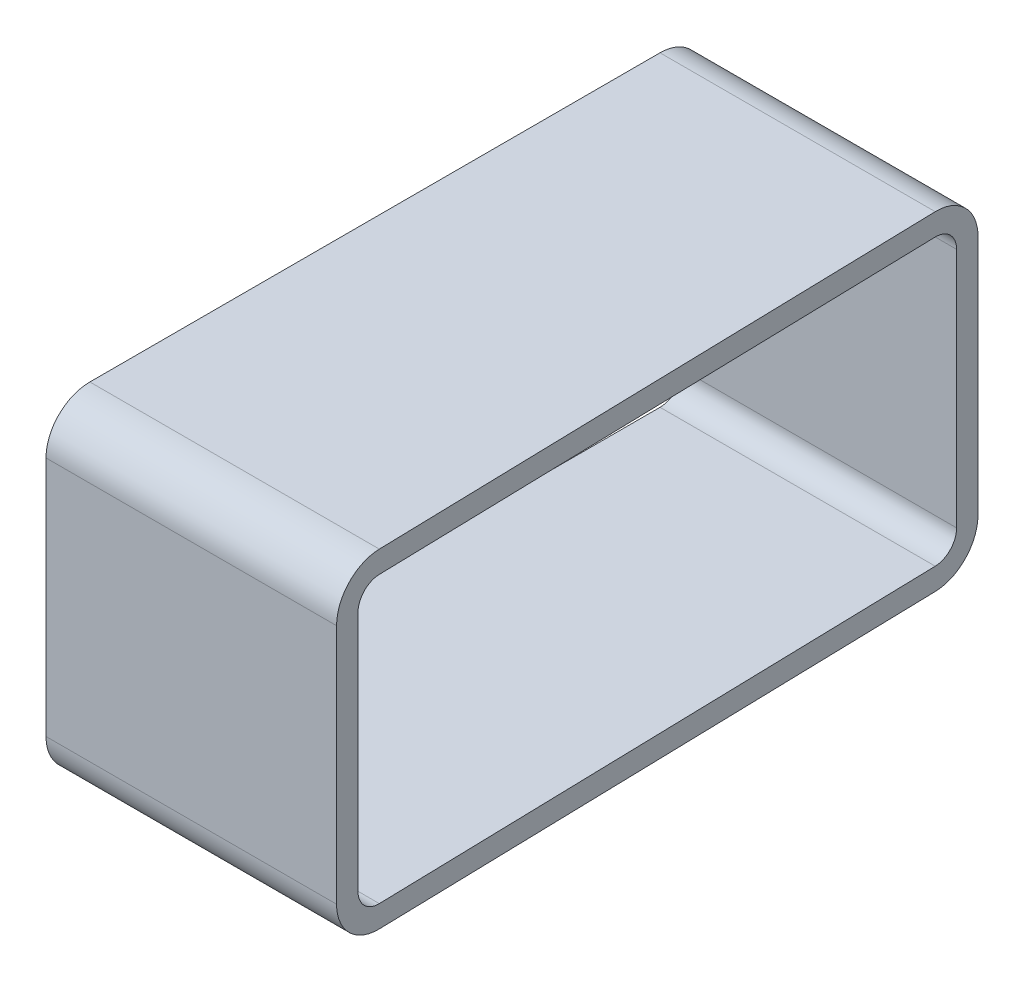
SolidWorks part; units mm, degrees
material "普通碳钢"
ref_plane "Front Plane" through (0, 0, 0) normal (0, 0, 1) x (1, 0, 0)
ref_plane "Top Plane" through (0, 0, 0) normal (0, 1, 0) x (1, 0, 0)
ref_plane "Right Plane" through (0, 0, 0) normal (1, 0, 0) x (0, 0, -1)
other "Configuration Table"
sketch "草图1" plane through (0, 0, 0) normal (0, 0, 1) x (1, 0, 0)
  line L0 (0, 0) -> (53, 0)
  dimension "D1" = 53
other "GB/6728-1986 rectangular hollow section 120 X 60 X 4(1)"
ref_plane "Plane1" through (0, 0, 0) normal (1, 0, 0) x (0, 1, 0)
sketch "Sketch1" plane through (0, 0, 0) normal (1, 0, 0) x (0, 1, 0)
  line L0 (-22, -56) -> (22, -56)
  line L1 (-26, -52) -> (-26, 52)
  line L2 (22, 56) -> (-22, 56)
  line L3 (26, 52) -> (26, -52)
  line L4 (-22, -60) -> (22, -60)
  line L5 (-30, -52) -> (-30, 52)
  line L6 (22, 60) -> (-22, 60)
  line L7 (30, 52) -> (30, -52)
  arc A0 (30, 52) -> (22, 60) centre (22, 52) ccw
  arc A1 (22, -60) -> (30, -52) centre (22, -52) ccw
  arc A2 (-30, -52) -> (-22, -60) centre (-22, -52) ccw
  arc A3 (-22, 60) -> (-30, 52) centre (-22, 52) ccw
  arc A4 (-22, 56) -> (-26, 52) centre (-22, 52) ccw
  arc A5 (26, 52) -> (22, 56) centre (22, 52) ccw
  arc A6 (22, -56) -> (26, -52) centre (22, -52) ccw
  arc A7 (-26, -52) -> (-22, -56) centre (-22, -52) ccw
  point P0 (0, 60)
  point P1 (30, 0)
  point P2 (0, -60)
  point P3 (-30, 0)
  point P4 (-30, 60)
  point P5 (30, 60)
  point P6 (30, -60)
  point P7 (-30, -60)
  point P8 (0, 0)
  point P33 (0, 0)
  dimension "D1" = 8
  dimension "Thickness" = 4
  dimension "V_leg" = 120
  dimension "H_leg" = 60
sketch "Sketch3" plane through (0, -30, 0) normal (0, -1, 0) x (1, 0, 0)
  line L0 (53, 60) -> (50, -60)
  line L1 (53, -60) -> (0, -60) construction
  line L2 (50, -60) -> (53, -60)
  line L3 (53, -60) -> (53, 60)
  dimension "D1" = 3
extrude "Cut-Extrude1" cut sketch "Sketch3" against normal through all both and the other way through all
